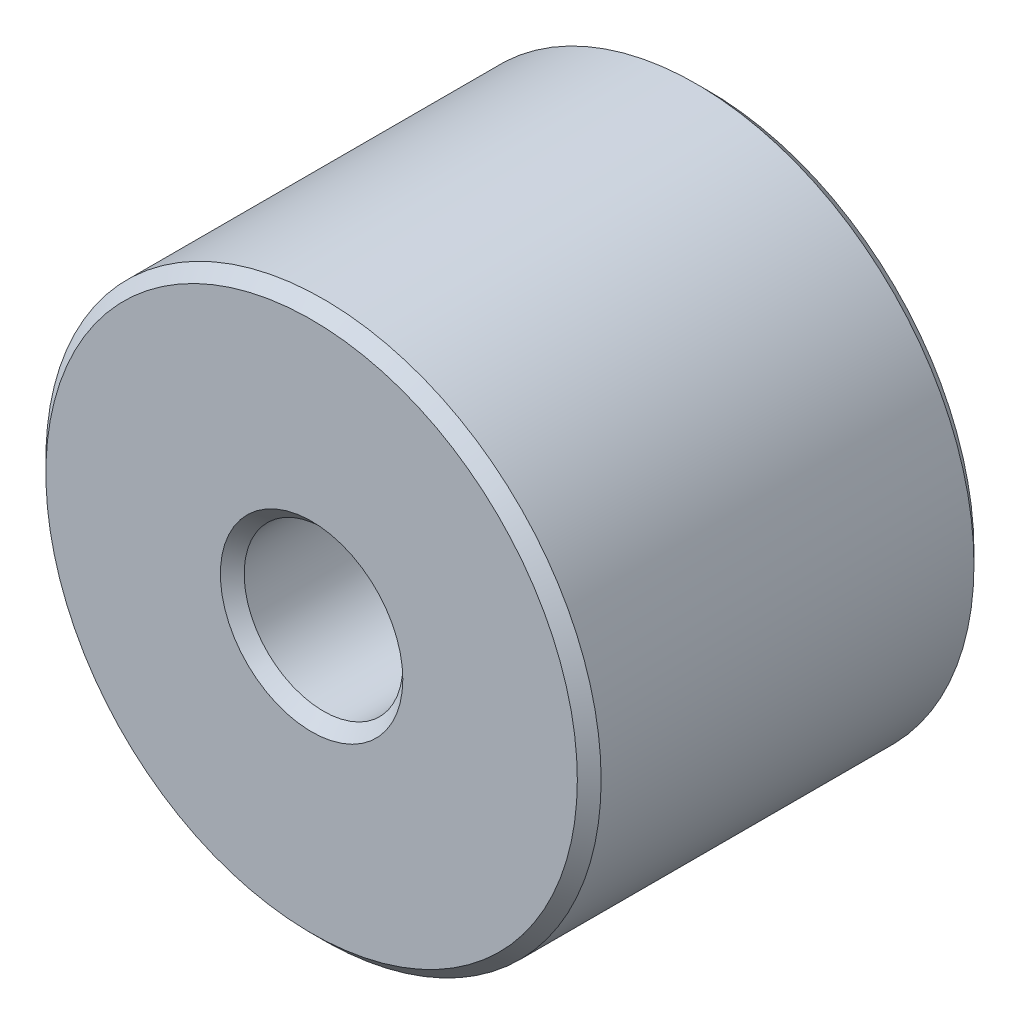
from build123d import *

# Parameters (mm, degrees)
SKETCH1_R           = 12.6
SKETCH1_R_2         = 3.6
BOSS_EXTRUDE1_DEPTH = 18
CHAMFER1_SIZE       = 0.54


with BuildPart() as part:
    # Sketch1 → Boss-Extrude1 (new body)
    with BuildSketch(Plane.XY):
        Circle(SKETCH1_R)
        Circle(SKETCH1_R_2, mode=Mode.SUBTRACT)
    extrude(amount=BOSS_EXTRUDE1_DEPTH)

    # Chamfer1
    chamfer1_edges = [part.edges().sort_by_distance(p)[0] for p in [
        (-12.6, 0, 0),
        (-12.6, 0, 18),
        (-3.6, 0, 0),
        (-3.6, 0, 18),
    ]]
    chamfer(chamfer1_edges, length=CHAMFER1_SIZE)


solid = part.part
